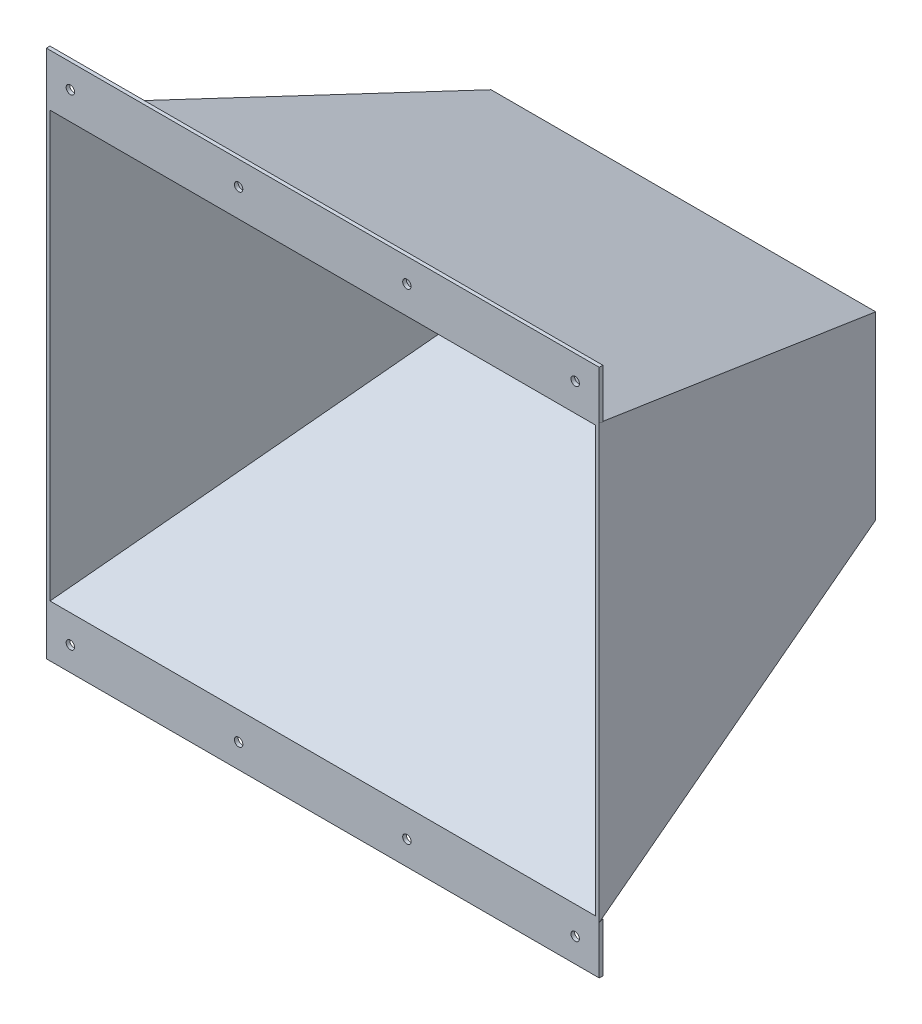
from build123d import *

# Parameters (mm, degrees)
SKETCH1_W                = 460
SKETCH1_H                = 360
BOSS_EXTRUDE1_DEPTH      = 300
CUT_EXTRUDE1_DEPTH       = 578.927331072
CUT_EXTRUDE3_DEPTH       = 302
SHELL1_T                 = -3
SKETCH7_W                = 315.23883128
SKETCH7_H                = 145.74311397
CUT_EXTRUDE4_DEPTH       = 417.544115311
SKETCH8_W                = 460
SKETCH8_H                = 40
BOSS_EXTRUDE2_DEPTH      = 3
BOSS_EXTRUDE3_REACH      = 524.015
SKETCH9_W                = 460
SKETCH9_H                = 3
SKETCH10_W               = 460
SKETCH10_H               = 40
BOSS_EXTRUDE4_DEPTH      = 3
BOSS_EXTRUDE5_REACH      = 552.364
SKETCH11_W               = 460
SKETCH11_H               = 3
F_7_0_7_DIAMETER_HOLE1_D = 7
LPATTERN1_COUNT          = 4
LPATTERN1_PITCH          = 140
MIRROR5_COPY_1_D         = 7
MIRROR5_COPY_2_D         = 7
MIRROR5_COPY_3_D         = 7


with BuildPart() as part:
    # Sketch1 → Boss-Extrude1 (new body)
    with BuildSketch(Plane.XY):
        Rectangle(SKETCH1_W, SKETCH1_H)
    extrude(amount=-BOSS_EXTRUDE1_DEPTH)

    # Sketch3 → Cut-Extrude1 (cut, through all)
    with BuildSketch(Plane(origin=(230, 0, 0), x_dir=(0, 0, -1), z_dir=(1, 0, 0))):
        Polygon((0, 180), (300, 75), (300, 180), align=None)
        Polygon((300, -180), (0, -180), (300, -75), align=None)
    extrude(amount=-CUT_EXTRUDE1_DEPTH, mode=Mode.SUBTRACT)

    # Sketch6 → Cut-Extrude3 (cut, symmetric)
    with BuildSketch(Plane(origin=(0, 0, 0), x_dir=(1, 0, 0), z_dir=(0, 1, 0))):
        Polygon((-230, 0), (-160, 300), (-230, 300), align=None)
        Polygon((230, 300), (230, 0), (160, 300), align=None)
    extrude(amount=CUT_EXTRUDE3_DEPTH, both=True, mode=Mode.SUBTRACT)

    # Shell1
    shell1_openings = [part.faces().sort_by_distance(p)[0] for p in [
        (0, 0, 0),
    ]]
    offset(amount=SHELL1_T, openings=shell1_openings, kind=Kind.INTERSECTION)

    # Sketch7 → Cut-Extrude4 (cut, through all)
    with BuildSketch(Plane.XY.offset(-297)):
        Rectangle(SKETCH7_W, SKETCH7_H)
    extrude(amount=-CUT_EXTRUDE4_DEPTH, mode=Mode.SUBTRACT)

    # Boss-Extrude3: up to this face of the body (flat: up to its plane)
    boss_extrude3_end = Plane(part.part.faces().sort_by_distance((0, -130.641025641, -141.025641026))[0])
    # Sketch9 → Boss-Extrude3 (add, up to the picked face)
    with BuildSketch(Plane(origin=(0, -180, 0), x_dir=(1, 0, 0), z_dir=(0, 1, 0)), mode=Mode.PRIVATE) as boss_extrude3_sk1:
        with Locations((0, 1.5)):
            Rectangle(SKETCH9_W, SKETCH9_H)
    boss_extrude3_tool1 = split(extrude(boss_extrude3_sk1.sketch, amount=BOSS_EXTRUDE3_REACH, mode=Mode.PRIVATE), bisect_by=boss_extrude3_end, keep=Keep.BOTH, mode=Mode.PRIVATE)


with BuildPart() as body_2:
    # Sketch8 → Boss-Extrude2 (new body)
    with BuildSketch(Plane.XY):
        with Locations((0, -200)):
            Rectangle(SKETCH8_W, SKETCH8_H)
    extrude(amount=-BOSS_EXTRUDE2_DEPTH)


with BuildPart() as part_1:
    add(part.part)

    add(body_2.part)  # Boss-Extrude3 merges body 2
    add(boss_extrude3_tool1.solids().sort_by(Axis((0, -180, -1.5), (0, 1, 0)))[0])

    # Boss-Extrude5: up to this face of the body (flat: up to its plane)
    boss_extrude5_end = Plane(part_1.part.faces().sort_by_distance((0, 130.641025641, -141.025641026))[0])
    # Sketch11 → Boss-Extrude5 (add, up to the picked face)
    with BuildSketch(Plane.XZ.offset(-180), mode=Mode.PRIVATE) as boss_extrude5_sk1:
        with Locations((0, -1.5)):
            Rectangle(SKETCH11_W, SKETCH11_H)
    boss_extrude5_tool1 = split(extrude(boss_extrude5_sk1.sketch, amount=BOSS_EXTRUDE5_REACH, mode=Mode.PRIVATE), bisect_by=boss_extrude5_end, keep=Keep.BOTH, mode=Mode.PRIVATE)


with BuildPart() as body_2_2:
    # Sketch10 → Boss-Extrude4 (new body)
    with BuildSketch(Plane.XY):
        with Locations((0, 200)):
            Rectangle(SKETCH10_W, SKETCH10_H)
    extrude(amount=-BOSS_EXTRUDE4_DEPTH)


with BuildPart() as part_2:
    add(part_1.part)

    add(body_2_2.part)  # Boss-Extrude5 merges body 2 2
    add(boss_extrude5_tool1.solids().sort_by(Axis((0, 180, -1.5), (0, -1, 0)))[0])

    # Ø7.0 (7) Diameter Hole1 (through all)
    with Locations(Plane.XY):
        with Locations((-210, 200)):
            f_7_0_7_diameter_hole1 = Hole(F_7_0_7_DIAMETER_HOLE1_D / 2)

    # LPattern1: Ø7.0 (7) Diameter Hole1 ×4
    with Locations(*[(i * LPATTERN1_PITCH, 0, 0) for i in range(1, LPATTERN1_COUNT)]):
        add(f_7_0_7_diameter_hole1, mode=Mode.SUBTRACT)

    # Mirror5: Ø7.0 (7) Diameter Hole1 across plane
    add(f_7_0_7_diameter_hole1.mirror(Plane.ZX), mode=Mode.SUBTRACT)

    # Mirror5 copy 1 (through all)
    with Locations(Plane(origin=(140, 0, 0), x_dir=(1, 0, 0), z_dir=(0, 0, 1))):
        with Locations((-210, -200)):
            Hole(MIRROR5_COPY_1_D / 2)

    # Mirror5 copy 2 (through all)
    with Locations(Plane(origin=(280, 0, 0), x_dir=(1, 0, 0), z_dir=(0, 0, 1))):
        with Locations((-210, -200)):
            Hole(MIRROR5_COPY_2_D / 2)

    # Mirror5 copy 3 (through all)
    with Locations(Plane(origin=(420, 0, 0), x_dir=(1, 0, 0), z_dir=(0, 0, 1))):
        with Locations((-210, -200)):
            Hole(MIRROR5_COPY_3_D / 2)


solid = part_2.part
